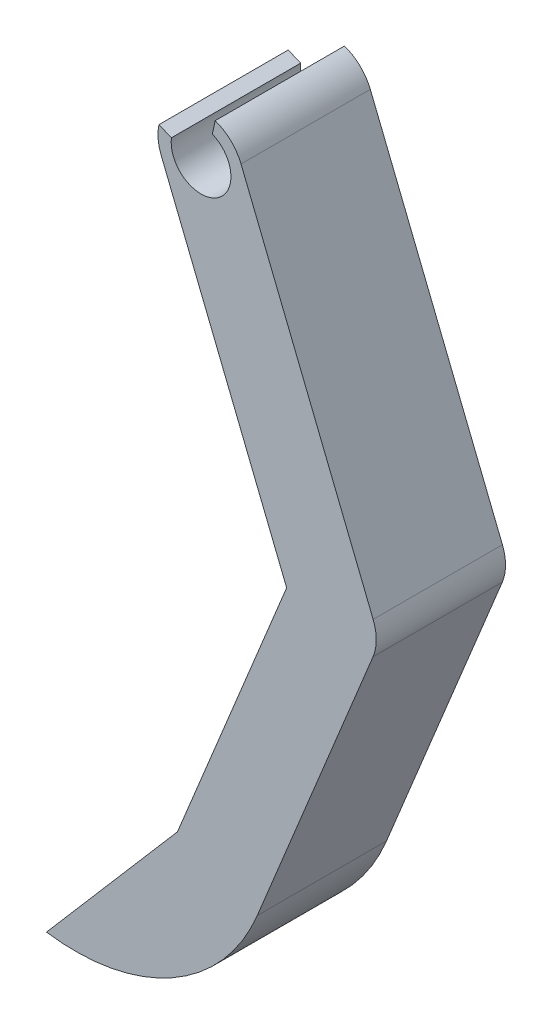
SolidWorks part; units mm, degrees
material "45"
ref_plane "Front Plane" through (0, 0, 0) normal (0, 0, 1) x (1, 0, 0)
ref_plane "Top Plane" through (0, 0, 0) normal (0, 1, 0) x (1, 0, 0)
ref_plane "Right Plane" through (0, 0, 0) normal (1, 0, 0) x (0, 0, -1)
sketch "Sketch1" plane through (0, 0, 0) normal (0, 0, 1) x (1, 0, 0)
  line L0 (15.4382, -15.8455) -> (21.5693, -31.0807) construction
  line L1 (17.2935, -15.0988) -> (23.4247, -30.3341)
  line L2 (13.5828, -16.5922) -> (19.714, -31.8274)
  line L3 (21.5693, -31.0807) -> (16.1951, -44.1701) construction
  line L4 (23.4195, -31.8404) -> (18.0453, -44.9297)
  line L5 (19.7192, -30.3211) -> (14.345, -43.4104)
  line L7 (14.0641, -15.6588) -> (13.4836, -15.4214)
  line L8 (15.963, -14.562) -> (16.0944, -13.9562)
  line L9 (14.345, -43.4104) -> (8.2662, -50.4817)
  arc A1 (14.0641, -15.6588) -> (15.963, -14.562) centre (15.4382, -15.8455) ccw
  arc A2 (17.2935, -15.0988) -> (16.0944, -13.9562) centre (15.4382, -15.8455) ccw
  arc A3 (19.714, -31.8274) -> (23.4247, -30.3341) centre (21.5693, -31.0807) ccw
  arc A4 (23.4195, -31.8404) -> (19.7192, -30.3211) centre (21.5693, -31.0807) ccw
  arc A6 (13.4836, -15.4214) -> (13.5828, -16.5922) centre (15.4382, -15.8455) ccw
  arc A7 (8.2662, -50.4817) -> (18.0453, -44.9297) centre (9.6144, -41.4681) ccw
  point P3 (18.5037, -23.4631)
  point P9 (18.8822, -37.6254)
  dimension "D1" = 2
  dimension "D3" = 80
  dimension "D4" = 2
  dimension "D5" = 2
extrude "Boss-Extrude1" add sketch "Sketch1" along normal blind 6 contours L7 A6 L2 L5 A4 L1 A2 L8 A1 | A3 A4 L5 L2 | L9 A7 L4 A3 L2 L5
